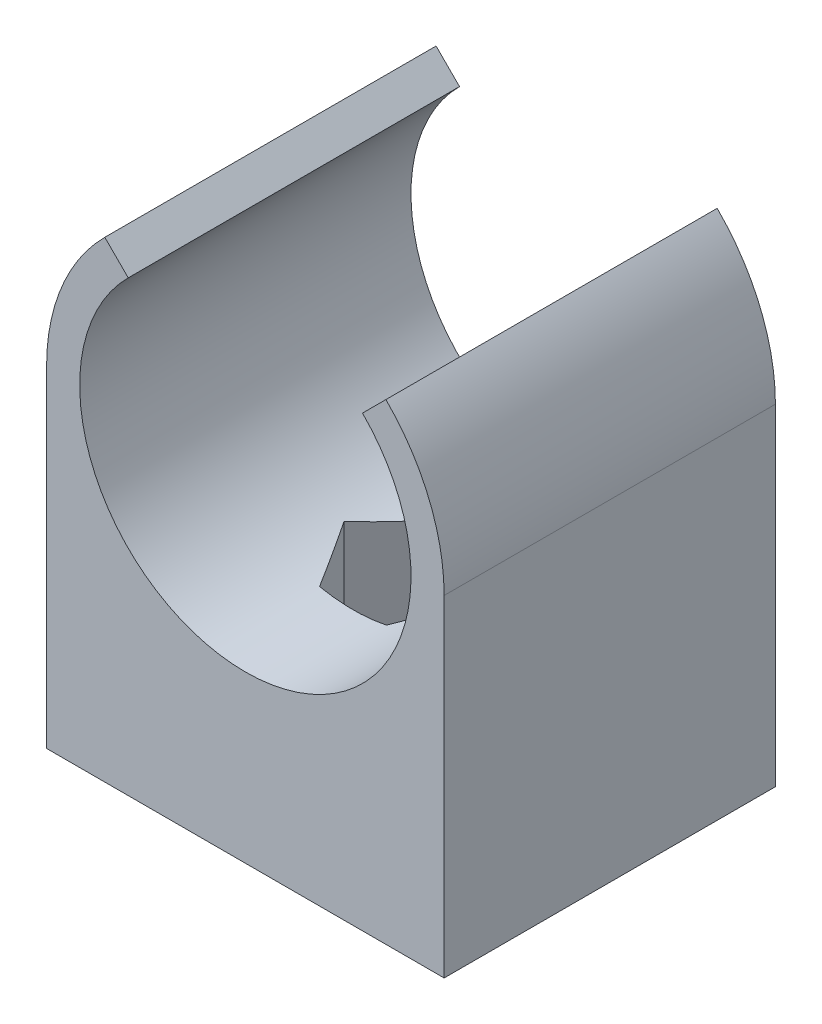
from build123d import *

# Parameters (mm, degrees)
EXTRUDE_1_DEPTH          = 20
HOLE_WIZARD_5_0_5_1_D    = 5
CUT_EXTRUDE_3_DEPTH      = 5
CUT_EXTRUDE_3_DEPTH_BACK = 5


with BuildPart() as part:
    # 草图1 → 凸台-拉伸1 (new body)
    with BuildSketch(Plane.XY):
        with BuildLine():
            Line((-12, 10), (-12, 20))
            ThreePointArc((-12, 20), (-11.08655439, 24.592201188), (-8.485281374, 28.485281374))
            Line((-8.485281374, 28.485281374), (-7.071067812, 27.071067812))
            ThreePointArc((-7.071067812, 27.071067812), (0, 10), (7.071067812, 27.071067812))
            Line((7.071067812, 27.071067812), (8.485281374, 28.485281374))
            ThreePointArc((8.485281374, 28.485281374), (11.08655439, 24.592201188), (12, 20))
            Line((12, 20), (12, 10))
            Line((12, 10), (12, 0))
            Line((12, 0), (-12, 0))
            Line((-12, 0), (-12, 10))
        make_face()
    extrude(amount=EXTRUDE_1_DEPTH)

    # Ø5.0 (5) 直径孔1 (through all)
    with Locations(Plane(origin=(0, 0, 0), x_dir=(-1, 0, 0), z_dir=(0, -1, 0))):
        with Locations((0, -10)):
            Hole(HOLE_WIZARD_5_0_5_1_D / 2)

    # 草图7 → 切除-拉伸3 (cut, two sides: drawn at the far end of the back side and taken through both)
    with BuildSketch(Plane(origin=(0, 10, 0), x_dir=(-1, 0, 0), z_dir=(0, -1, 0)).offset(-CUT_EXTRUDE_3_DEPTH_BACK)):
        Polygon((4.041451884, -10), (2.020725942, -6.5), (-2.020725942, -6.5), (-4.041451884, -10), (-2.020725942, -13.5), (2.020725942, -13.5), align=None)
    extrude(amount=CUT_EXTRUDE_3_DEPTH + CUT_EXTRUDE_3_DEPTH_BACK, mode=Mode.SUBTRACT)


solid = part.part
